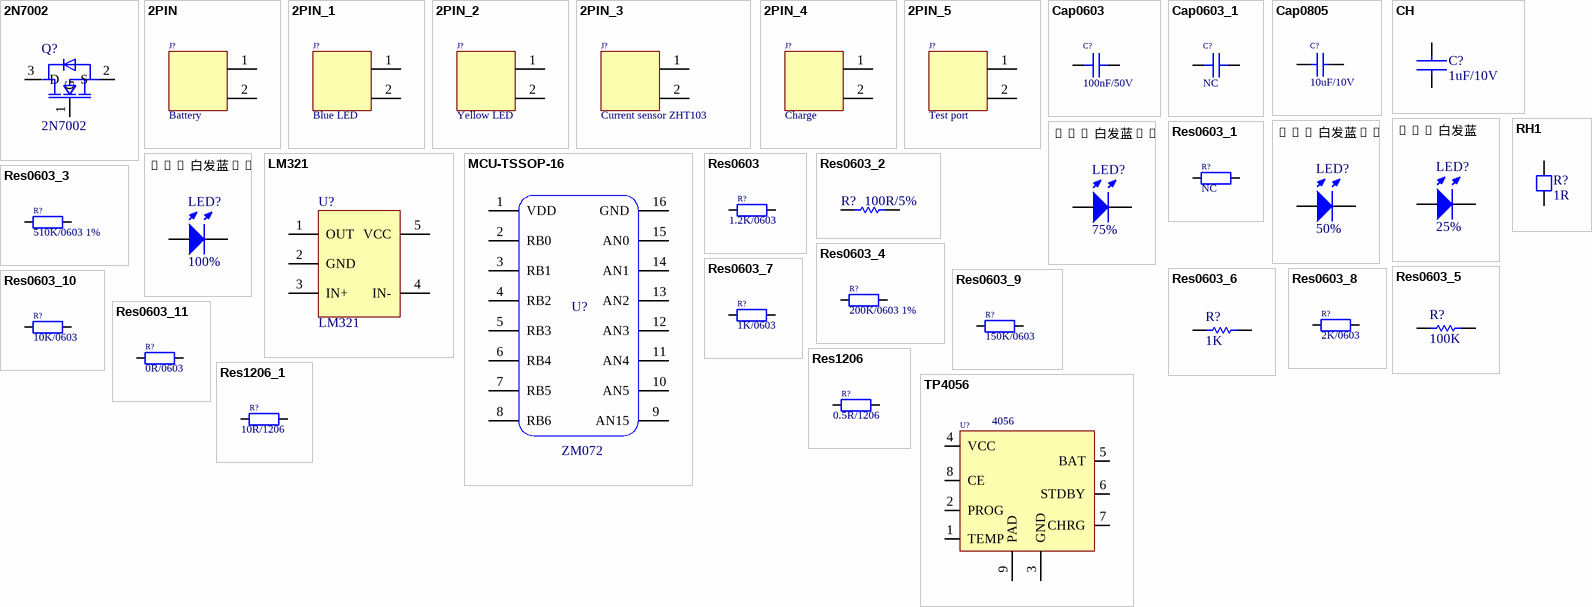
[diagram p0: symbols 2N7002 to TP4056]
# Altium schematic symbol library MISC84244-4.SchLib: 33 symbols
Pins are listed as number, name and electrical type; pins without a type are passive.


## 2N7002
designator Q?
SMD MOSFET
footprint SOT23-3L (SMD MOS)
footprint SOT23-3 (SMD IC/MOS*)
pins: 1 G, 2 S, 3 D

## 2PIN
designator J?, comment Battery
DC jack right-angle 90° pitch 2.0; 物料名称: DC jack 2PIN; 封装: pitch 2.0 90° right-angle THT
footprint GH1.25-2PIN立贴带扣耐温260℃ (Vertical SMD, latched, rated 260℃)
pins: 1, 2

## 2PIN_1
designator J?, comment Blue LED
DC jack right-angle 90° pitch 2.0; 物料名称: DC jack 2PIN; 封装: pitch 2.0 90° right-angle THT
footprint GH1.25-2PIN立贴带扣耐温260℃ (Vertical SMD, latched, rated 260℃)
pins: 1, 2

## 2PIN_2
designator J?, comment Yellow LED
DC jack right-angle 90° pitch 2.0; 物料名称: DC jack 2PIN; 封装: pitch 2.0 90° right-angle THT
footprint GH1.25-2PIN立贴带扣耐温260℃ (Vertical SMD, latched, rated 260℃)
pins: 1, 2

## 2PIN_3
designator J?, comment Current sensor ZHT103
DC jack right-angle 90° pitch 2.0; 物料名称: DC jack 2PIN; 封装: pitch 2.0 90° right-angle THT
footprint IND-TH_L18.2-W10.2-P12.00-D0.9_ZHT103
pins: 1, 2

## 2PIN_4
designator J?, comment Charge
DC jack right-angle 90° pitch 2.0; 物料名称: DC jack 2PIN; 封装: pitch 2.0 90° right-angle THT
footprint HY2.0WT-2A/P 立贴带扣耐温260℃ (Horizontal SMD connector)
pins: 1, 2

## 2PIN_5
designator J?, comment Test port
DC jack right-angle 90° pitch 2.0; 物料名称: DC jack 2PIN; 封装: pitch 2.0 90° right-angle THT
footprint HY2.0WT-2A/P 立贴带扣耐温260℃ (Horizontal SMD connector)
pins: 1, 2

## Cap0603
designator C?, comment 100nF/50V
footprint C0603A (SMD capacitor)
pins: 1, 2

## Cap0603_1
designator C?, comment NC
footprint C0603A (SMD capacitor)
pins: 1, 2

## Cap0805
designator C?, comment 10uF/10V
SMD capacitor; 规格: 0805-16V-106-X7R
footprint C0805 (SMD capacitor C0805)
footprint C0805A (SMD capacitor)
pins: 1, 2

## CH
designator C?, comment 1uF/10V
footprint 0603HD
footprint 0805B
footprint 1206H
footprint 0603C
footprint 0603DC
footprint C0603A (SMD capacitor)
pins: 1, 2
2 alternate drawings of the same symbol

## LED 白发蓝
designator LED?, comment 25%
SMD LED; 规格: 0603-diffused-ice blue
footprint 0603-LED-CB
footprint LED-DIP-2
footprint LED0603A
footprint LED-0603
footprint 0603-LED
footprint LED0603A (SMD LED)
pins: 1, 2

## LED 白发蓝_1
designator LED?, comment 50%
SMD LED; 规格: 0603-diffused-ice blue
footprint 0603-LED-CB
footprint LED-DIP-2
footprint LED0603A
footprint LED-0603
footprint 0603-LED
footprint LED0603A (SMD LED)
pins: 1, 2

## LED 白发蓝_2
designator LED?, comment 75%
SMD LED; 规格: 0603-diffused-ice blue
footprint 0603-LED-CB
footprint LED-DIP-2
footprint LED0603A
footprint LED-0603
footprint 0603-LED
footprint LED0603A (SMD LED)
pins: 1, 2

## LED 白发蓝_3
designator LED?, comment 100%
SMD LED; 规格: 0603-diffused-ice blue
footprint 0603-LED-CB
footprint LED-DIP-2
footprint LED0603A
footprint LED-0603
footprint 0603-LED
footprint LED0603A (SMD LED)
pins: 1, 2

## LM321
designator U?
footprint SOT-23-5
footprint SOT23-5A (SMD IC)
pins: 1 OUT, 2 GND, 3 IN+, 4 IN-, 5 VCC

## MCU-TSSOP-16
designator U?, comment ZM072
footprint TSSOP-20
footprint TSSOP-16A
footprint TSSOP-16(间距0.65mm) (SMD IC)
footprint SOP16L
pins: 1 VDD, 2 RB0, 3 RB1, 4 RB2, 5 RB3, 6 RB4, 7 RB5, 8 RB6, 9 AN15, 10 AN5, 11 AN4, 12 AN3, 13 AN2, 14 AN1, 15 AN0, 16 GND

## Res0603
designator R?, comment 1.2K/0603
SMD resistor; 规格: 0603
footprint R0603
footprint R0603A (SMD resistor)
pins: 1, 2

## Res0603_1
designator R?, comment NC
SMD resistor; 规格: 0603
footprint R0603
footprint R0603A (SMD resistor)
pins: 1, 2

## Res0603_2
designator R?, comment 100R/5%
SMD resistor; 规格: 0603
footprint 0603 (1608)
footprint 0402 (1005)
footprint 1206 (3216)
footprint 2512 (6432)
footprint 0201 (0603)
footprint 0805 (2012)
footprint 1210 (3528  3225)
footprint R0603
footprint R0603
footprint 0603D
footprint R0603A (SMD resistor)
pins: 1, 2

## Res0603_3
designator R?, comment 510K/0603 1%
SMD resistor; 规格: 0603
footprint R0603
footprint R0603A (SMD resistor)
pins: 1, 2

## Res0603_4
designator R?, comment 200K/0603 1%
SMD resistor; 规格: 0603
footprint R0603
footprint R0603A (SMD resistor)
pins: 1, 2

## Res0603_5
designator R?, comment 100K
SMD resistor; 规格: 0603
footprint 0603 (1608)
footprint 0402 (1005)
footprint 1206 (3216)
footprint 2512 (6432)
footprint 0201 (0603)
footprint 0805 (2012)
footprint 1210 (3528  3225)
footprint R0603
footprint R0603
footprint 0603D
footprint R0603A (SMD resistor)
pins: 1, 2

## Res0603_6
designator R?, comment 1K
SMD resistor; 规格: 0603
footprint 0603 (1608)
footprint 0402 (1005)
footprint 1206 (3216)
footprint 2512 (6432)
footprint 0201 (0603)
footprint 0805 (2012)
footprint 1210 (3528  3225)
footprint R0603
footprint R0603
footprint 0603D
footprint R0603A (SMD resistor)
pins: 1, 2

## Res0603_7
designator R?, comment 1K/0603
SMD resistor; 规格: 0603
footprint R0603
footprint R0603A (SMD resistor)
pins: 1, 2

## Res0603_8
designator R?, comment 2K/0603
SMD resistor; 规格: 0603
footprint R0603
footprint R0603A (SMD resistor)
pins: 1, 2

## Res0603_9
designator R?, comment 150K/0603
SMD resistor; 规格: 0603
footprint R0603
footprint R0603A (SMD resistor)
pins: 1, 2

## Res0603_10
designator R?, comment 10K/0603
SMD resistor; 规格: 0603
footprint R0603
footprint R0603A (SMD resistor)
pins: 1, 2

## Res0603_11
designator R?, comment 0R/0603
SMD resistor; 规格: 0603
footprint R0603
footprint R0603A (SMD resistor)
pins: 1, 2

## Res1206
designator R?, comment 0.5R/1206
SMD resistor; 规格: 0603-43.2K-1%
footprint R1206
footprint R1206A (SMD resistor)
pins: 1, 2

## Res1206_1
designator R?, comment 10R/1206
SMD resistor; 规格: 0603-43.2K-1%
footprint R1206
footprint R1206A (SMD resistor)
pins: 1, 2

## RH1
designator R?, comment 1R
footprint 0603D
footprint 0805H
footprint 1206H
footprint 0603C
footprint R0603A (SMD resistor)
pins: 1, 2
2 alternate drawings of the same symbol

## TP4056
designator U?, comment 4056
Charger IC; 规格: ESOP-8; 物料名称: Charger IC 4056
footprint ESOP-8
footprint ESOP-8L (SMD MOS/IC)
pins: 1 TEMP, 2 PROG, 3 GND, 4 VCC, 5 BAT, 6 STDBY, 7 CHRG, 8 CE, 9 PAD